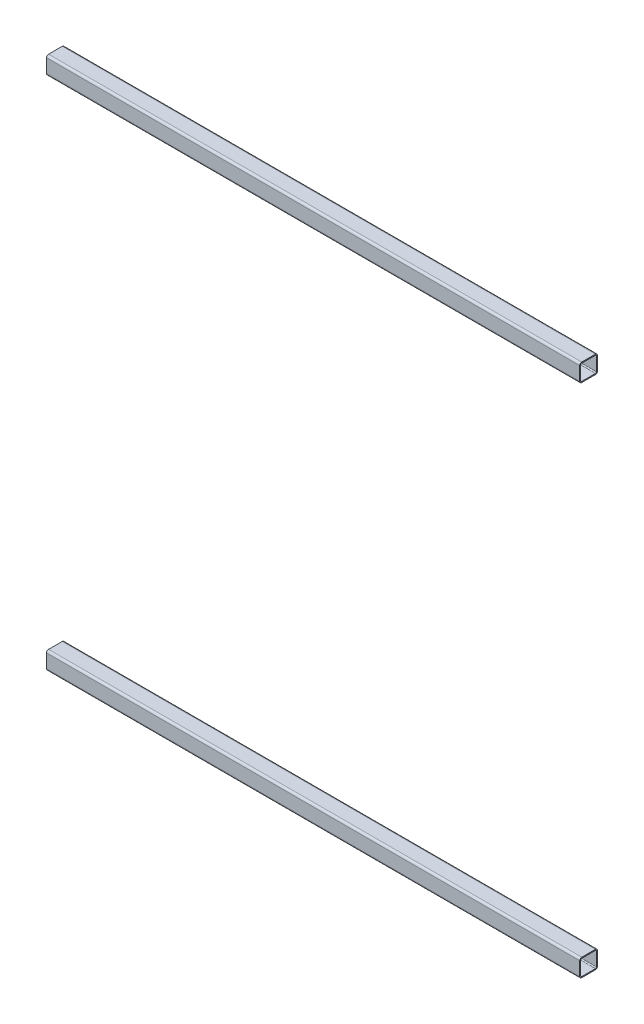
from build123d import *

# Parameters (mm, degrees)
SQUARE_TUBE_40_X_40_X_2_3_1_DEPTH   = 1200
SQUARE_TUBE_40_X_40_X_2_3_1_2_DEPTH = 1200


with BuildPart() as part:
    # Sketch11 → Square Tube 40 X 40 X 2.3(1) (new body)
    with BuildSketch(Plane.YZ):
        with BuildLine():
            Line((-15.4, -20), (15.4, -20))
            ThreePointArc((15.4, -20), (18.652691193, -18.652691193), (20, -15.4))
            Line((20, -15.4), (20, 15.4))
            ThreePointArc((20, 15.4), (18.652691193, 18.652691193), (15.4, 20))
            Line((15.4, 20), (-15.4, 20))
            ThreePointArc((-15.4, 20), (-18.652691193, 18.652691193), (-20, 15.4))
            Line((-20, 15.4), (-20, -15.4))
            ThreePointArc((-20, -15.4), (-18.652691193, -18.652691193), (-15.4, -20))
        make_face()
        with BuildLine():
            Line((-15.4, -17.7), (15.4, -17.7))
            ThreePointArc((15.4, -17.7), (17.026345597, -17.026345597), (17.7, -15.4))
            Line((17.7, -15.4), (17.7, 15.4))
            ThreePointArc((17.7, 15.4), (17.026345597, 17.026345597), (15.4, 17.7))
            Line((15.4, 17.7), (-15.4, 17.7))
            ThreePointArc((-15.4, 17.7), (-17.026345597, 17.026345597), (-17.7, 15.4))
            Line((-17.7, 15.4), (-17.7, -15.4))
            ThreePointArc((-17.7, -15.4), (-17.026345597, -17.026345597), (-15.4, -17.7))
        make_face(mode=Mode.SUBTRACT)
    extrude(amount=SQUARE_TUBE_40_X_40_X_2_3_1_DEPTH)


with BuildPart() as body_2:
    # Sketch11 on segment 2 (carried to segment 2) → Square Tube 40 X 40 X 2.3_1 2 (new body)
    with BuildSketch(Plane(origin=(0, 1160, 0), x_dir=(0, 1, 0), z_dir=(1, 0, 0))):
        with BuildLine():
            Line((-15.4, -20), (15.4, -20))
            ThreePointArc((15.4, -20), (18.652691193, -18.652691193), (20, -15.4))
            Line((20, -15.4), (20, 15.4))
            ThreePointArc((20, 15.4), (18.652691193, 18.652691193), (15.4, 20))
            Line((15.4, 20), (-15.4, 20))
            ThreePointArc((-15.4, 20), (-18.652691193, 18.652691193), (-20, 15.4))
            Line((-20, 15.4), (-20, -15.4))
            ThreePointArc((-20, -15.4), (-18.652691193, -18.652691193), (-15.4, -20))
        make_face()
        with BuildLine():
            Line((-15.4, -17.7), (15.4, -17.7))
            ThreePointArc((15.4, -17.7), (17.026345597, -17.026345597), (17.7, -15.4))
            Line((17.7, -15.4), (17.7, 15.4))
            ThreePointArc((17.7, 15.4), (17.026345597, 17.026345597), (15.4, 17.7))
            Line((15.4, 17.7), (-15.4, 17.7))
            ThreePointArc((-15.4, 17.7), (-17.026345597, 17.026345597), (-17.7, 15.4))
            Line((-17.7, 15.4), (-17.7, -15.4))
            ThreePointArc((-17.7, -15.4), (-17.026345597, -17.026345597), (-15.4, -17.7))
        make_face(mode=Mode.SUBTRACT)
    extrude(amount=SQUARE_TUBE_40_X_40_X_2_3_1_2_DEPTH)


solid = Compound([part.part, body_2.part])
